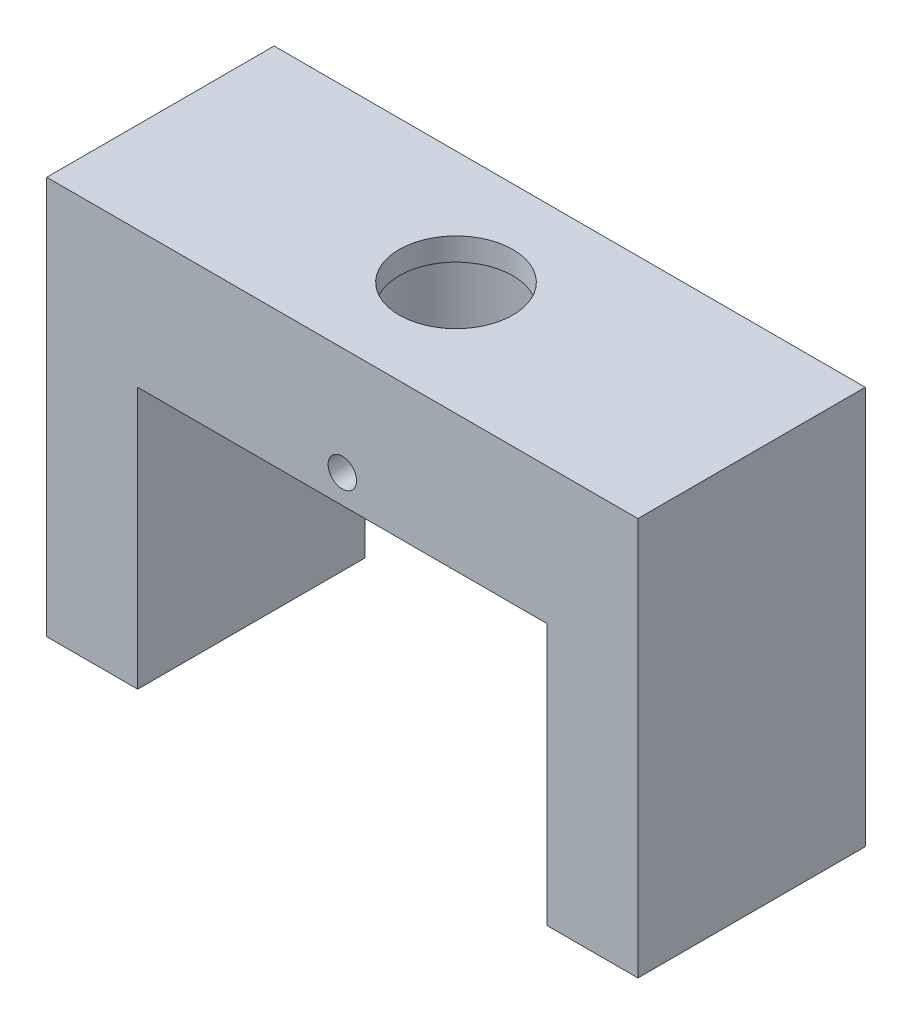
SolidWorks part; units mm, degrees
ref_plane "Front Plane" through (0, 0, 0) normal (0, 0, 1) x (1, 0, 0)
ref_plane "Top Plane" through (0, 0, 0) normal (0, 1, 0) x (1, 0, 0)
ref_plane "Right Plane" through (0, 0, 0) normal (1, 0, 0) x (0, 0, -1)
sketch "Sketch1" plane through (0, 0, 0) normal (0, 0, 1) x (1, 0, 0)
  line L0 (-18, -6.7408) -> (-26, -6.7408)
  line L3 (-26, -6.7408) -> (-26, 28.2592)
  line L4 (-26, 28.2592) -> (26, 28.2592)
  line L5 (0, 16.2592) -> (0, 0) construction
  line L6 (-18, -6.7408) -> (-18, 16.2592)
  line L7 (-18, 16.2592) -> (18, 16.2592)
  line L9 (18, -6.7408) -> (18, 16.2592)
  line L10 (26, -6.7408) -> (26, 28.2592)
  line L13 (18, -6.7408) -> (26, -6.7408)
  point P7 (-26, 10.7592)
  dimension "D2" = 35
  dimension "D4" = 18
  dimension "D5" = 12
  dimension "D6" = 8
extrude "Boss-Extrude1" add sketch "Sketch1" along normal mid plane 20
sketch "Sketch3" plane through (0, 28.2592, 0) normal (0, 1, 0) x (1, 0, 0)
  circle A0 centre (0, 0) radius 5
  dimension "D1" = 10
extrude "Cut-Extrude2" cut sketch "Sketch3" against normal blind 27
sketch "Sketch5" plane through (0, -6.7408, 0) normal (0, -1, 0) x (1, 0, 0)
  line L0 (18, -10) -> (26, -10) construction
  line L1 (18, 10) -> (26, 10) construction
  line L2 (0, 0) -> (0, 12.0207) construction
  line L3 (26, 10) -> (26, -10) construction
  circle A0 centre (22, 6) radius 1.5
  circle A1 centre (22, -6) radius 1.5
  circle A2 centre (-22, -6) radius 1.5
  circle A3 centre (-22, 6) radius 1.5
  dimension "D1" = 4
  dimension "D3" = 4
  dimension "D4" = 4
  dimension "D2" = 4
extrude "Cut-Extrude4" cut sketch "Sketch5" against normal blind 10
hole_wizard "M4 Tapped Hole1" positions "Sketch7" profile "Sketch8" tap size "M4" standard "GB"
sketch "Sketch7" plane through (0, -6.7408, 0) normal (0, -1, 0) x (-1, 0, 0)
  point P0 (-22, 6)
  point P3 (-22, -6)
  point P6 (22, 6)
  point P9 (22, -6)
sketch "Sketch8" plane through (22, -6.7408, -6) normal (1, 0, 0) x (0, 0, -1)
  line L0 (0, 0) -> (0, 10.9914)
  line L1 (0, 10.9914) -> (1.65, 10)
  line L2 (1.65, 10) -> (1.65, 0)
  line L5 (1.65, 0) -> (0, 0)
  line L10 (0, 10.9914) -> (-1.65, 10) construction
  line L11 (0, -6.35) -> (0, 107.95) construction
  dimension "螺纹孔钻头直径" = 3.3
  dimension "螺纹孔钻头深度" = 10
  dimension "导头角度" = 118
cosmetic thread "CosmeticThread1" parameters "D1"=8, "D2"=4
cosmetic thread "CosmeticThread2" parameters "D1"=8, "D2"=4
cosmetic thread "CosmeticThread3" parameters "D1"=8, "D2"=4
cosmetic thread "CosmeticThread4" parameters "D1"=8, "D2"=4
sketch "Sketch9" plane through (0, 16.2592, 0) normal (0, -1, 0) x (1, 0, 0)
  circle A0 centre (0, 0) radius 7.5
extrude "Cut-Extrude5" cut sketch "Sketch9" against normal blind 10
sketch "Sketch10" plane through (0, 0, 10) normal (0, 0, 1) x (1, 0, 0)
  line L3 (0, 16.2592) -> (0, 18.7592) construction
  line L4 (-18, 16.2592) -> (18, 16.2592) construction
  dimension "D1" = 2.5
hole_wizard "M3 Tapped Hole2" positions "Sketch13" profile "Sketch14" tap size "M3" standard "GB"
sketch "Sketch13" plane through (0, 0, 10) normal (0, 0, 1) x (1, 0, 0)
  point P0 (0, 18.7592)
sketch "Sketch14" plane through (0, 18.7592, 10) normal (1, 0, 0) x (0, -1, 0)
  line L0 (0, 0) -> (0, 2.5)
  line L1 (0, 2.5) -> (1.25, 2.5)
  line L2 (1.25, 2.5) -> (1.25, 0)
  line L5 (1.25, 0) -> (0, 0)
  line L11 (0, -6.35) -> (0, 107.95) construction
  dimension "通孔螺纹孔钻头直径" = 2.5
  dimension "通孔螺纹孔钻头深度" = 2.5
cosmetic thread "CosmeticThread6" parameters "D2"=3
sketch "Sketch15" plane through (0, 16.2592, 0) normal (0, -1, 0) x (1, 0, 0)
  circle A0 centre (0, 0) radius 10
hole_wizard "M3 Tapped Hole3" positions "Sketch16" profile "Sketch17" tap size "M3" standard "GB"
sketch "Sketch16" plane through (0, 16.2592, 0) normal (0, -1, 0) x (-1, 0, 0)
  circle A0 centre (0, 0) radius 10 construction
  point P0 (10, 0)
  point P4 (-10, 0)
sketch "Sketch17" plane through (-10, 16.2592, 0) normal (1, 0, 0) x (0, 0, -1)
  line L0 (0, 0) -> (0, 10.7511)
  line L1 (0, 10.7511) -> (1.25, 10)
  line L2 (1.25, 10) -> (1.25, 0)
  line L5 (1.25, 0) -> (0, 0)
  line L10 (0, 10.7511) -> (-1.25, 10) construction
  line L11 (0, -6.35) -> (0, 107.95) construction
  dimension "螺纹孔钻头直径" = 2.5
  dimension "螺纹孔钻头深度" = 10
  dimension "导头角度" = 118
cosmetic thread "CosmeticThread7" parameters "D1"=10, "D2"=3
cosmetic thread "CosmeticThread8" parameters "D1"=10, "D2"=3
